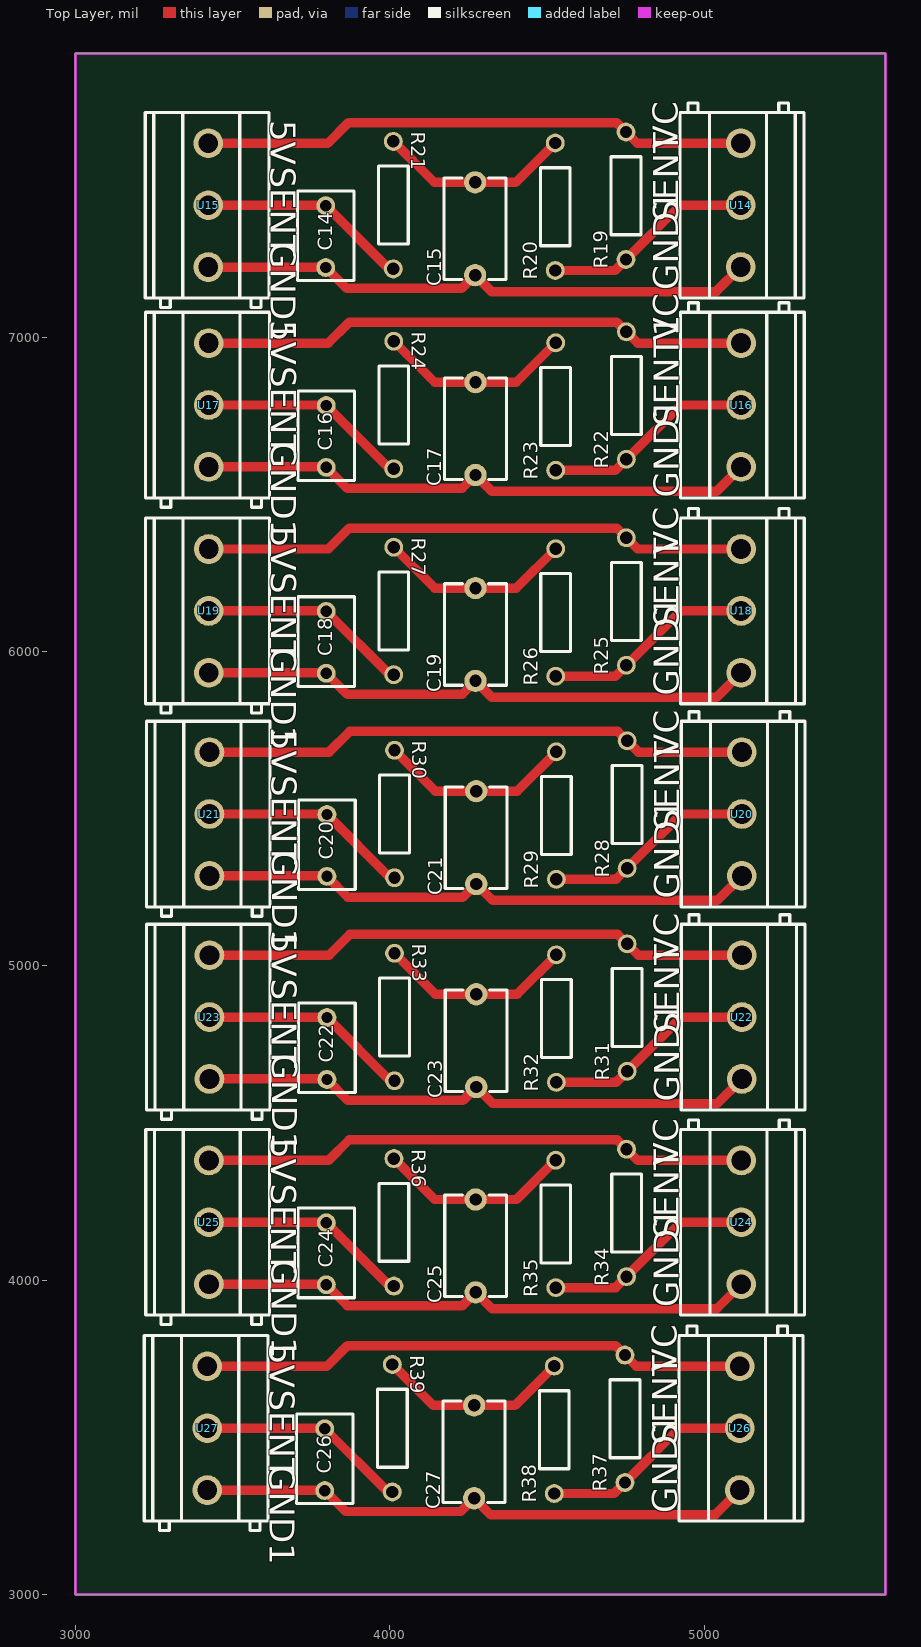
[diagram p0: Top Layer view]
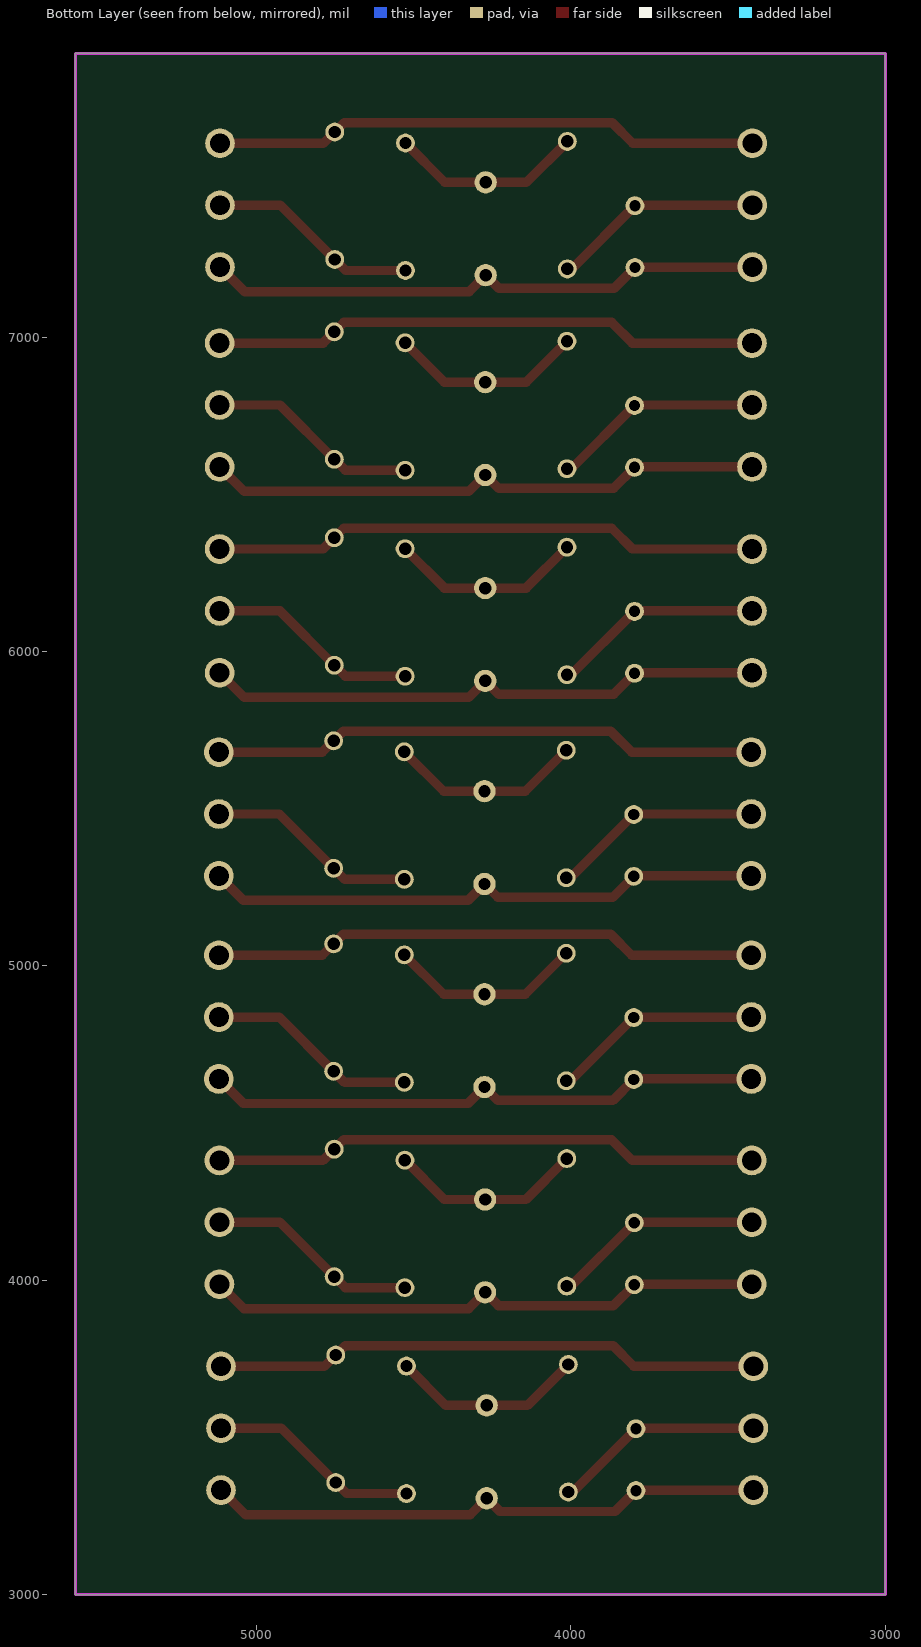
[diagram p1: Bottom Layer view, seen from below]
# Altium PCB MISC52118.pcbdoc
Units mil, origin at the board's own origin, x right, y up, seen from the top; angles counter-clockwise.
Board outline 2576.47 x 4902.76 mil, 2 copper layers (Top Layer, Bottom Layer), stack 62.206 mil thick; 49 components, 35 nets, 112 pads, 0 vias.

## Layer stack, top to bottom
Top Solder Mask Layer: solder mask 0.394, Dk 3.3
Top Layer: signal copper 1.379
Dielectric1: surface 59.449, FR4, Dk 4.5
Bottom Layer: signal copper 1.378
Bottom Solder Mask Layer: solder mask 0.394, Dk 3.3

## Board outline
3000,7902.76 3000,3000 5576.47,3000 5576.47,7902.76

## Design rules (kind name [scope] priority, off if disabled: settings)
BoardOutlineClearance copperThickness2oz_1 [All] p2 off: genericclearance=7.99 ignorepadtopadclearanceinfootprint=FALSE except(0: Arc-SplitContinuation Track-SplitContinuation SMDPad-SplitContinuation THPad-SplitContinuation Via-SplitContinuation Fill-SplitContinuation Region-SplitContinuation Poly-SplitContinuation Text-SplitContinuation Hole-SplitContinuation; 5.98: Arc-CutoutEdge Track-CutoutEdge SMDPad-CutoutEdge THPad-CutoutEdge Via-CutoutEdge Text-CutoutEdge; 6.89: Hole-OutlineEdge Hole-CutoutEdge; 10: Poly-OutlineEdge Poly-CutoutEdge; 11.81: Arc-OutlineEdge Track-OutlineEdge SMDPad-OutlineEdge THPad-OutlineEdge Via-OutlineEdge Fill-OutlineEdge Region-OutlineEdge Text-OutlineEdge Fill-CutoutEdge Region-CutoutEdge)
BoardOutlineClearance Plane_innerPlane_1 [All] p4 off: genericclearance=4.02 ignorepadtopadclearanceinfootprint=FALSE except(0: Arc-SplitContinuation Track-SplitContinuation SMDPad-SplitContinuation THPad-SplitContinuation Via-SplitContinuation Fill-SplitContinuation Region-SplitContinuation Poly-SplitContinuation Text-SplitContinuation Hole-SplitContinuation; 5.98: Arc-CutoutEdge Track-CutoutEdge SMDPad-CutoutEdge THPad-CutoutEdge Via-CutoutEdge Text-CutoutEdge; 6.89: Hole-OutlineEdge Hole-CutoutEdge; 10: Poly-OutlineEdge Poly-CutoutEdge; 11.81: Arc-OutlineEdge Track-OutlineEdge SMDPad-OutlineEdge THPad-OutlineEdge Via-OutlineEdge Fill-OutlineEdge Region-OutlineEdge Text-OutlineEdge Fill-CutoutEdge Region-CutoutEdge)
BoardOutlineClearance Copper_copperRegion_1 [All] p6 off: genericclearance=4.02 ignorepadtopadclearanceinfootprint=FALSE except(0: Arc-SplitContinuation Track-SplitContinuation SMDPad-SplitContinuation THPad-SplitContinuation Via-SplitContinuation Fill-SplitContinuation Region-SplitContinuation Poly-SplitContinuation Text-SplitContinuation Hole-SplitContinuation; 5.98: Arc-CutoutEdge Track-CutoutEdge SMDPad-CutoutEdge THPad-CutoutEdge Via-CutoutEdge Text-CutoutEdge; 6.89: Hole-OutlineEdge Hole-CutoutEdge; 10: Poly-OutlineEdge Poly-CutoutEdge; 11.81: Arc-OutlineEdge Track-OutlineEdge SMDPad-OutlineEdge THPad-OutlineEdge Via-OutlineEdge Fill-OutlineEdge Region-OutlineEdge Text-OutlineEdge Fill-CutoutEdge Region-CutoutEdge)
BoardOutlineClearance copperThickness1oz_1 [All] p8: genericclearance=4.02 ignorepadtopadclearanceinfootprint=FALSE except(0: Arc-SplitContinuation Track-SplitContinuation SMDPad-SplitContinuation THPad-SplitContinuation Via-SplitContinuation Fill-SplitContinuation Region-SplitContinuation Poly-SplitContinuation Text-SplitContinuation Hole-SplitContinuation; 5.98: Arc-CutoutEdge Track-CutoutEdge SMDPad-CutoutEdge THPad-CutoutEdge Via-CutoutEdge Text-CutoutEdge; 6.89: Hole-OutlineEdge Hole-CutoutEdge; 10: Poly-OutlineEdge Poly-CutoutEdge; 11.81: Arc-OutlineEdge Track-OutlineEdge SMDPad-OutlineEdge THPad-OutlineEdge Via-OutlineEdge Fill-OutlineEdge Region-OutlineEdge Text-OutlineEdge Fill-CutoutEdge Region-CutoutEdge)
Clearance copperThickness2oz [All] p1 off: gap=7.99 ignorepadtopadclearanceinfootprint=FALSE except(5.98: SMDPad-Track SMDPad-SMDPad THPad-Track SMDPad-THPad THPad-THPad Track-Via SMDPad-Via THPad-Via Via-Via Fill-SMDPad Region-SMDPad Fill-THPad Region-THPad Fill-Via Region-Via Fill-Fill Fill-Region Region-Region Arc-Track Arc-SMDPad Arc-THPad Arc-Via Fill-Arc Region-Arc Arc-Arc Text-Track SMDPad-Text Text-THPad Text-Via Fill-Text Region-Text Arc-Text Text-Text; 6.89: Hole-Track Hole-SMDPad Hole-THPad Hole-Via Fill-Hole Region-Hole Hole-Arc Hole-Text; 10: Poly-Track Poly-SMDPad Poly-THPad Poly-Via Poly-Fill Poly-Region Poly-Poly Poly-Arc Poly-Text Poly-Hole; 11.81: Fill-Track Region-Track)
Clearance Plane_innerPlane [All] p3 off: gap=4.02 ignorepadtopadclearanceinfootprint=FALSE except(5.98: SMDPad-Track SMDPad-SMDPad THPad-Track SMDPad-THPad THPad-THPad Track-Via SMDPad-Via THPad-Via Via-Via Fill-SMDPad Region-SMDPad Fill-THPad Region-THPad Fill-Via Region-Via Fill-Fill Fill-Region Region-Region Arc-Track Arc-SMDPad Arc-THPad Arc-Via Fill-Arc Region-Arc Arc-Arc Text-Track SMDPad-Text Text-THPad Text-Via Fill-Text Region-Text Arc-Text Text-Text; 6.89: Hole-Track Hole-SMDPad Hole-THPad Hole-Via Fill-Hole Region-Hole Hole-Arc Hole-Text; 10: Poly-Track Poly-SMDPad Poly-THPad Poly-Via Poly-Fill Poly-Region Poly-Poly Poly-Arc Poly-Text Poly-Hole; 11.81: Fill-Track Region-Track)
Clearance Copper_copperRegion [All] p5 off: gap=4.02 ignorepadtopadclearanceinfootprint=FALSE except(5.98: SMDPad-Track SMDPad-SMDPad THPad-Track SMDPad-THPad THPad-THPad Track-Via SMDPad-Via THPad-Via Via-Via Fill-SMDPad Region-SMDPad Fill-THPad Region-THPad Fill-Via Region-Via Fill-Fill Fill-Region Region-Region Arc-Track Arc-SMDPad Arc-THPad Arc-Via Fill-Arc Region-Arc Arc-Arc Text-Track SMDPad-Text Text-THPad Text-Via Fill-Text Region-Text Arc-Text Text-Text; 6.89: Hole-Track Hole-SMDPad Hole-THPad Hole-Via Fill-Hole Region-Hole Hole-Arc Hole-Text; 10: Poly-Track Poly-SMDPad Poly-THPad Poly-Via Poly-Fill Poly-Region Poly-Poly Poly-Arc Poly-Text Poly-Hole; 11.81: Fill-Track Region-Track)
Clearance copperThickness1oz [All] p7: gap=4.02 ignorepadtopadclearanceinfootprint=FALSE except(5.98: SMDPad-Track SMDPad-SMDPad THPad-Track SMDPad-THPad THPad-THPad Track-Via SMDPad-Via THPad-Via Via-Via Fill-SMDPad Region-SMDPad Fill-THPad Region-THPad Fill-Via Region-Via Fill-Fill Fill-Region Region-Region Arc-Track Arc-SMDPad Arc-THPad Arc-Via Fill-Arc Region-Arc Arc-Arc Text-Track SMDPad-Text Text-THPad Text-Via Fill-Text Region-Text Arc-Text Text-Text; 6.89: Hole-Track Hole-SMDPad Hole-THPad Hole-Via Fill-Hole Region-Hole Hole-Arc Hole-Text; 10: Poly-Track Poly-SMDPad Poly-THPad Poly-Via Poly-Fill Poly-Region Poly-Poly Poly-Arc Poly-Text Poly-Hole; 11.81: Fill-Track Region-Track)
DiffPairsRouting differentialPair [All] p1: maxlimit=6 minlimit=6 mostfreqgap=6 toplayer_minwidth=5 toplayer_prefwidth=10 toplayer_maxwidth=100 toplayer_mingap=6 toplayer_prefgap=6 toplayer_maxgap=6 bottomlayer_minwidth=5 bottomlayer_prefwidth=10 bottomlayer_maxwidth=100 bottomlayer_mingap=6 bottomlayer_prefgap=6 bottomlayer_maxgap=6 maxuncoupledlength=10
HoleToHoleClearance otherClearance [All] p1: gap=11.81 allowstackedmicrovias=TRUE
Length netLength [All] p1: minlimit=0 maxlimit=0
PasteMaskExpansion pasteMaskExpansion [All] p1: expansion=0
PlaneConnect innerPlane [All] p1: planeconnectstyle=Relief reliefexpansion=20 reliefentries=4 reliefconductorwidth=10 reliefairgap=10
PolygonConnect copperRegion [All] p1: connectstyle=Relief reliefconductorwidth=10 reliefentries=4 polygonreliefangle="90 Angle" airgapwidth=10 via.connectstyle=Relief via.reliefconductorwidth=10 via.reliefentries=4 via.polygonreliefangle="90 Angle" via.airgapwidth=10
RoutingVias viaSize [All] p1: holewidth=12.01 width=24.02 viastyle="Through Hole" minholewidth=11.81 minwidth=19.68 maxholewidth=248.03 maxwidth=393.7
SolderMaskExpansion solderMaskExpansion [IsVia] p1: expansion=-1000 istentingtop=TRUE
SolderMaskExpansion solderMaskExpansion [All] p2: expansion=2.01 istentingtop=FALSE
Width copperThickness2oz_2 [All] p1 off: maxlimit=100 minlimit=8 preferedwidth=10
Width copperThickness1oz_2 [All] p2: maxlimit=100 minlimit=5 preferedwidth=30

## Components (designator, comment, footprint, x,y, rotation, side; value= is the part's Value field where it differs from the comment)
C14 "220pF" CAP-TH_L7.2-W4.5-P5.00-D0.5 3796.47,7320 r90 top
C15 "2.2nF" CAP-TH_L8.0-W5.0-P7.50-D1.0 4271.47,7345 r90 top
C16 "220pF" CAP-TH_L7.2-W4.5-P5.00-D0.5 3797.76,6684.27 r90 top
C17 "2.2nF" CAP-TH_L8.0-W5.0-P7.50-D1.0 4272.76,6709.27 r90 top
C18 "220pF" CAP-TH_L7.2-W4.5-P5.00-D0.5 3797.76,6029.27 r90 top
C19 "2.2nF" CAP-TH_L8.0-W5.0-P7.50-D1.0 4272.76,6054.27 r90 top
C20 "220pF" CAP-TH_L7.2-W4.5-P5.00-D0.5 3800.08,5383.15 r90 top
C21 "2.2nF" CAP-TH_L8.0-W5.0-P7.50-D1.0 4275.08,5408.15 r90 top
C22 "220pF" CAP-TH_L7.2-W4.5-P5.00-D0.5 3800.08,4737.24 r90 top
C23 "2.2nF" CAP-TH_L8.0-W5.0-P7.50-D1.0 4275.08,4762.24 r90 top
C24 "220pF" CAP-TH_L7.2-W4.5-P5.00-D0.5 3798.28,4084.27 r90 top
C25 "2.2nF" CAP-TH_L8.0-W5.0-P7.50-D1.0 4273.28,4109.27 r90 top
C26 "220pF" CAP-TH_L7.2-W4.5-P5.00-D0.5 3793.28,3429.27 r90 top
C27 "2.2nF" CAP-TH_L8.0-W5.0-P7.50-D1.0 4268.28,3454.27 r90 top
R19 "51kΩ" Res_1/4W 4751.47,7450 r90 top
R20 "390Ω" Res_1/4W 4526.47,7415 r90 top
R21 "3.6kΩ" Res_1/4W 4011.47,7420 r270 top
R22 "51kΩ" Res_1/4W 4752.76,6814.27 r90 top
R23 "390Ω" Res_1/4W 4527.76,6779.27 r90 top
R24 "3.6kΩ" Res_1/4W 4012.76,6784.27 r270 top
R25 "51kΩ" Res_1/4W 4752.76,6159.27 r90 top
R26 "390Ω" Res_1/4W 4527.76,6124.27 r90 top
R27 "3.6kΩ" Res_1/4W 4012.76,6129.27 r270 top
R28 "51kΩ" Res_1/4W 4755.08,5513.15 r90 top
R29 "390Ω" Res_1/4W 4530.08,5478.15 r90 top
R30 "3.6kΩ" Res_1/4W 4015.08,5483.15 r270 top
R31 "51kΩ" Res_1/4W 4755.08,4867.24 r90 top
R32 "390Ω" Res_1/4W 4530.08,4832.24 r90 top
R33 "3.6kΩ" Res_1/4W 4015.08,4837.24 r270 top
R34 "51kΩ" Res_1/4W 4753.28,4214.27 r90 top
R35 "390Ω" Res_1/4W 4528.28,4179.27 r90 top
R36 "3.6kΩ" Res_1/4W 4013.28,4184.27 r270 top
R37 "51kΩ" Res_1/4W 4748.28,3559.27 r90 top
R38 "390Ω" Res_1/4W 4523.28,3524.27 r90 top
R39 "3.6kΩ" Res_1/4W 4008.28,3529.27 r270 top
U14 "KF128L-5.0-3P" CONN-TH_3P-P5.00_KF128L-5.0-3P 5116.47,7420 r90 top
U15 "KF128L-5.0-3P" CONN-TH_3P-P5.00_KF128L-5.0-3P 3422.87,7420 r270 top
U16 "KF128L-5.0-3P" CONN-TH_3P-P5.00_KF128L-5.0-3P 5117.76,6784.27 r90 top
U17 "KF128L-5.0-3P" CONN-TH_3P-P5.00_KF128L-5.0-3P 3424.16,6784.27 r270 top
U18 "KF128L-5.0-3P" CONN-TH_3P-P5.00_KF128L-5.0-3P 5117.76,6129.27 r90 top
U19 "KF128L-5.0-3P" CONN-TH_3P-P5.00_KF128L-5.0-3P 3424.16,6129.27 r270 top
U20 "KF128L-5.0-3P" CONN-TH_3P-P5.00_KF128L-5.0-3P 5120.08,5483.15 r90 top
U21 "KF128L-5.0-3P" CONN-TH_3P-P5.00_KF128L-5.0-3P 3426.47,5483.15 r270 top
U22 "KF128L-5.0-3P" CONN-TH_3P-P5.00_KF128L-5.0-3P 5120.08,4837.24 r90 top
U23 "KF128L-5.0-3P" CONN-TH_3P-P5.00_KF128L-5.0-3P 3426.47,4837.24 r270 top
U24 "KF128L-5.0-3P" CONN-TH_3P-P5.00_KF128L-5.0-3P 5118.28,4184.27 r90 top
U25 "KF128L-5.0-3P" CONN-TH_3P-P5.00_KF128L-5.0-3P 3424.68,4184.27 r270 top
U26 "KF128L-5.0-3P" CONN-TH_3P-P5.00_KF128L-5.0-3P 5113.28,3529.27 r90 top
U27 "KF128L-5.0-3P" CONN-TH_3P-P5.00_KF128L-5.0-3P 3419.68,3529.27 r270 top

## Footprints (in the part's own frame and the unit in brackets; to place one, negate y for a bottom-side part, rotate by r counter-clockwise, add the part's x,y. Pads: shape width x height; smd on the part's side, far side on the other; paste and mask are expansions set on the pad)
CAP-TH_L7.2-W4.5-P5.00-D0.5 [mil]
  round 60 hole 36 paste+0 mask+1.97: 1(-98.43,0) 2(98.43,0)
  silkscreen extent -140,-90 145,90
CAP-TH_L8.0-W5.0-P7.50-D1.0 [mm]
  round 1.8 hole 1: 1(-3.75,0) 2(3.75,0)
  silkscreen extent -4.1,-2.5 4.1,2.5
CONN-TH_3P-P5.00_KF128L-5.0-3P [mm]
  round 2.4 hole 1.6: 1(-5,0) 2(0,0) 3(5,0)
  silkscreen extent -7.5,-5.1 8.26,4.9
Res_1/4W [mil]
  round 60 hole 39.37 paste+0 mask+2: 1(-202.76,0) 2(202.76,0)
  silkscreen extent -124,-47 124,47

## Nets (pads, with @x,y where several pads share a name; then routed paths per layer and width w, separated by ;. In a path a pad name is that pad's centre, name@x,y a point inside that pad or via, vN(x,y) a via of type N, cw(c..) or ccw(c..) an arc to the next point about the centre after c; other vN are vias at no path point)
$1N3242: R19.1 R20.1 U14.2 | length 676.1
  Top Layer w30: R20.1 4716.47,7212.24 R19.1 4924.23,7420 U14.2
$1N3246: R19.2 U14.3 U15.1 | length 1748.2
  Top Layer w30: U15.1 3803.32,7616.85 3869.23,7682.76 4721.47,7682.76 R19.2 4787.38,7616.85 U14.3
$1N3258: C15.2 R20.2 R21.1 | length 620.7
  Top Layer w30: R21.1 4141.59,7492.64 C15.2 4401.35,7492.64 R20.2
$1N3264: C14.2 R21.2 U15.2 | length 672.6
  Top Layer w30: U15.2 3794.9,7420 C14.2 3997.66,7217.24 R21.2
$1N3270: C14.1 C15.1 U14.1 U15.3 | length 1793.4
  Top Layer w30: U15.3 3794.9,7223.15 C14.1 3863.05,7155 4229.11,7155 C15.1 4323.83,7145 5038.32,7145 U14.1
$1N3641: R22.1 R23.1 U16.2 | length 676.1
  Top Layer w30: R23.1 4717.76,6576.51 R22.1 4925.52,6784.27 U16.2
$1N3644: R22.2 U16.3 U17.1 | length 1748.2
  Top Layer w30: U17.1 3804.61,6981.12 3870.52,7047.03 4722.76,7047.03 R22.2 4788.67,6981.12 U16.3
$1N3649: C17.2 R23.2 R24.1 | length 620.7
  Top Layer w30: R24.1 4142.88,6856.91 C17.2 4402.64,6856.91 R23.2
$1N3652: C16.2 R24.2 U17.2 | length 672.6
  Top Layer w30: U17.2 3796.18,6784.27 C16.2 3998.94,6581.51 R24.2
$1N3655: C16.1 C17.1 U16.1 U17.3 | length 1793.4
  Top Layer w30: U17.3 3796.18,6587.42 C16.1 3864.33,6519.27 4230.4,6519.27 C17.1 4325.12,6509.27 5039.61,6509.27 U16.1
$1N3884: R25.1 R26.1 U18.2 | length 676.1
  Top Layer w30: R26.1 4717.76,5921.51 R25.1 4925.52,6129.27 U18.2
$1N3887: R25.2 U18.3 U19.1 | length 1748.2
  Top Layer w30: U19.1 3804.61,6326.12 3870.52,6392.03 4722.76,6392.03 R25.2 4788.67,6326.12 U18.3
$1N3892: C19.2 R26.2 R27.1 | length 620.7
  Top Layer w30: R27.1 4142.88,6201.91 C19.2 4402.64,6201.91 R26.2
$1N3895: C18.2 R27.2 U19.2 | length 672.6
  Top Layer w30: U19.2 3796.18,6129.27 C18.2 3998.94,5926.51 R27.2
$1N3898: C18.1 C19.1 U18.1 U19.3 | length 1793.4
  Top Layer w30: U19.3 3796.18,5932.42 C18.1 3864.33,5864.27 4230.4,5864.27 C19.1 4325.12,5854.27 5039.61,5854.27 U18.1
$1N4127: R28.1 R29.1 U20.2 | length 676.1
  Top Layer w30: R29.1 4720.08,5275.39 R28.1 4927.84,5483.15 U20.2
$1N4130: R28.2 U20.3 U21.1 | length 1748.2
  Top Layer w30: U21.1 3806.93,5680 3872.84,5745.91 4725.08,5745.91 R28.2 4790.99,5680 U20.3
$1N4135: C21.2 R29.2 R30.1 | length 620.7
  Top Layer w30: R30.1 4145.2,5555.79 C21.2 4404.96,5555.79 R29.2
$1N4138: C20.2 R30.2 U21.2 | length 672.6
  Top Layer w30: U21.2 3798.5,5483.15 C20.2 4001.26,5280.39 R30.2
$1N4141: C20.1 C21.1 U20.1 U21.3 | length 1793.4
  Top Layer w30: U21.3 3798.5,5286.3 C20.1 3866.65,5218.15 4232.72,5218.15 C21.1 4327.44,5208.15 5041.93,5208.15 U20.1
$1N5033: R31.1 R32.1 U22.2 | length 676.1
  Top Layer w30: R32.1 4720.08,4629.48 R31.1 4927.84,4837.24 U22.2
$1N5036: C23.2 R32.2 R33.1 | length 620.7
  Top Layer w30: R33.1 4145.2,4909.88 C23.2 4404.96,4909.88 R32.2
$1N5039: C25.2 R35.2 R36.1 | length 620.7
  Top Layer w30: R36.1 4143.4,4256.91 C25.2 4403.16,4256.91 R35.2
$1N5042: R34.2 U24.3 U25.1 | length 1748.2
  Top Layer w30: U25.1 3805.13,4381.12 3871.04,4447.03 4723.28,4447.03 R34.2 4789.19,4381.12 U24.3
$1N5047: C24.1 C25.1 U24.1 U25.3 | length 1793.4
  Top Layer w30: U25.3 3796.71,3987.42 C24.1 3864.86,3919.27 4230.92,3919.27 C25.1 4325.64,3909.27 5040.13,3909.27 U24.1
$1N5054: R34.1 R35.1 U24.2 | length 676.1
  Top Layer w30: R35.1 4718.28,3976.51 R34.1 4926.04,4184.27 U24.2
$1N5057: C24.2 R36.2 U25.2 | length 672.6
  Top Layer w30: U25.2 3796.71,4184.27 C24.2 3999.47,3981.51 R36.2
$1N5060: C26.1 C27.1 U26.1 U27.3 | length 1793.4
  Top Layer w30: U27.3 3791.71,3332.42 C26.1 3859.86,3264.27 4225.92,3264.27 C27.1 4320.64,3254.27 5035.13,3254.27 U26.1
$1N5067: C27.2 R38.2 R39.1 | length 620.7
  Top Layer w30: R39.1 4138.4,3601.91 C27.2 4398.16,3601.91 R38.2
$1N5070: R37.1 R38.1 U26.2 | length 676.1
  Top Layer w30: R38.1 4713.28,3321.51 R37.1 4921.04,3529.27 U26.2
$1N5073: C26.2 R39.2 U27.2 | length 672.6
  Top Layer w30: U27.2 3791.71,3529.27 C26.2 3994.47,3326.51 R39.2
$1N5076: R37.2 U26.3 U27.1 | length 1748.2
  Top Layer w30: U27.1 3800.13,3726.12 3866.04,3792.03 4718.28,3792.03 R37.2 4784.19,3726.12 U26.3
$1N5099: C22.1 C23.1 U22.1 U23.3 | length 1793.4
  Top Layer w30: U23.3 3798.5,4640.39 C22.1 3866.65,4572.24 4232.72,4572.24 C23.1 4327.44,4562.24 5041.93,4562.24 U22.1
$1N5106: R31.2 U22.3 U23.1 | length 1748.2
  Top Layer w30: U23.1 3806.93,5034.09 3872.84,5100 4725.08,5100 R31.2 4790.99,5034.09 U22.3
$1N5111: C22.2 R33.2 U23.2 | length 672.6
  Top Layer w30: U23.2 3798.5,4837.24 C22.2 4001.26,4634.48 R33.2

## Keep-outs
Board Outline Layer:
  the board outline again, w10

## Silkscreen, mask and mechanical layers (free items; w line width, h text height)
Top Silkscreen Layer:
  text "5V" at 3621.47,7690 h78.74 r270
  text "VC" at 4916.47,7600 h78.74 r90
  text "SENT" at 3621.47,7542.6 h78.74 r270
  text "SENT" at 4917.87,7367.35 h78.74 r90
  text "GND1" at 3622.1,7302.7 h78.74 r270
  text "GND1" at 4917.87,7150 h78.74 r90
  text "5V" at 3622.76,7054.27 h78.74 r270
  text "VC" at 4917.76,6989.27 h78.74 r90
  text "SENT" at 3622.76,6906.87 h78.74 r270
  text "SENT1" at 4919.16,6716.77 h78.74 r90
  text "GND1" at 3623.39,6666.97 h78.74 r270
  text "GND1" at 4919.16,6489.27 h78.74 r90
  text "5V" at 3622.76,6399.27 h78.74 r270
  text "VC" at 4917.76,6309.27 h78.74 r90
  text "SENT" at 3622.76,6251.87 h78.74 r270
  text "SENT" at 4919.16,6076.62 h78.74 r90
  text "GND1" at 3623.39,6011.97 h78.74 r270
  text "GND1" at 4919.16,5859.27 h78.74 r90
  text "5V" at 3625.08,5753.15 h78.74 r270
  text "VC" at 4920.08,5663.15 h78.74 r90
  text "SENT" at 3625.08,5605.75 h78.74 r270
  text "SENT" at 4921.47,5430.5 h78.74 r90
  text "GND1" at 3625.71,5365.85 h78.74 r270
  text "GND1" at 4921.47,5213.15 h78.74 r90
  text "5V" at 3625.08,5107.24 h78.74 r270
  text "VC" at 4920.08,5017.24 h78.74 r90
  text "SENT" at 3625.08,4959.84 h78.74 r270
  text "SENT" at 4921.47,4784.59 h78.74 r90
  text "GND1" at 3625.71,4719.94 h78.74 r270
  text "GND1" at 4921.47,4567.24 h78.74 r90
  text "5V" at 3623.28,4454.27 h78.74 r270
  text "VC" at 4918.28,4364.27 h78.74 r90
  text "SENT" at 3623.28,4306.87 h78.74 r270
  text "SENT" at 4919.68,4131.62 h78.74 r90
  text "GND1" at 3623.91,4066.97 h78.74 r270
  text "GND1" at 4919.68,3914.27 h78.74 r90
  text "5V" at 3618.28,3799.27 h78.74 r270
  text "VC" at 4913.28,3709.27 h78.74 r90
  text "SENT" at 3618.28,3651.87 h78.74 r270
  text "SENT" at 4914.68,3476.62 h78.74 r90
  text "GND1" at 3618.91,3411.97 h78.74 r270
  text "GND1" at 4914.68,3259.27 h78.74 r90